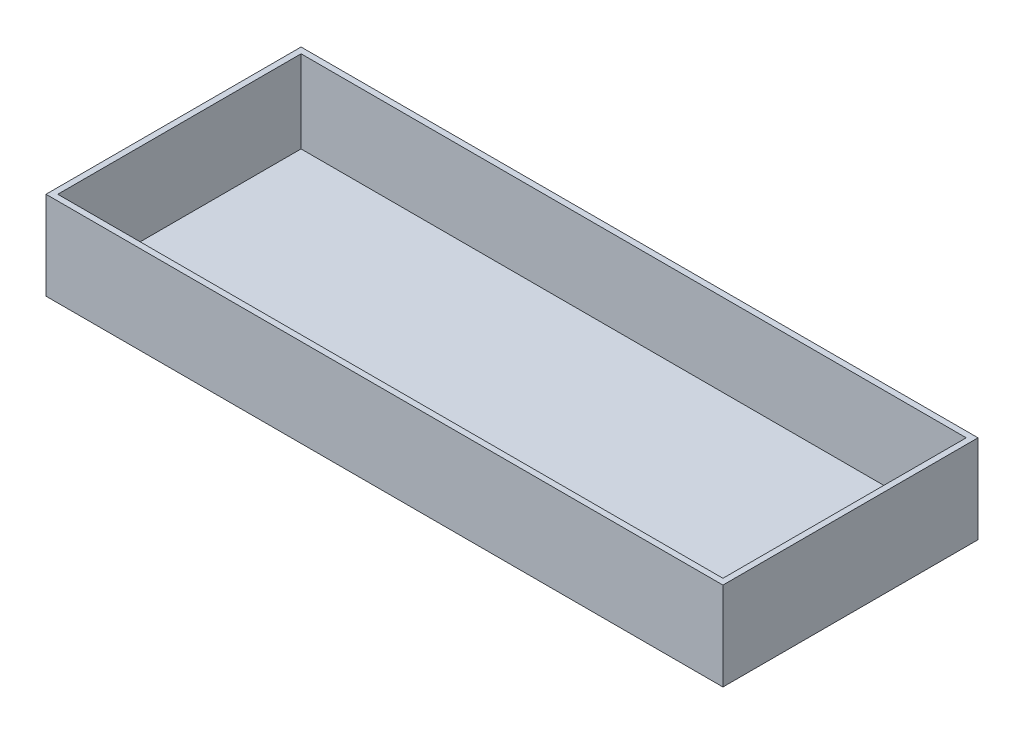
SolidWorks part; units mm, degrees
ref_plane "Front Plane" through (0, 0, 0) normal (0, 0, 1) x (1, 0, 0)
ref_plane "Top Plane" through (0, 0, 0) normal (0, 1, 0) x (1, 0, 0)
ref_plane "Right Plane" through (0, 0, 0) normal (1, 0, 0) x (0, 0, -1)
sketch "Sketch1" plane through (0, 0, 0) normal (0, 1, 0) x (1, 0, 0)
  line L1 (-345, 130) -> (345, 130)
  line L2 (-345, 130) -> (-345, -130)
  line L3 (-345, -130) -> (345, -130)
  line L4 (345, 130) -> (345, -130)
  line L5 (-345, 130) -> (345, -130) construction
  line L6 (-345, -130) -> (345, 130) construction
  point P0 (0, 0)
  dimension "D1" = 260
  dimension "D2" = 690
extrude "Boss-Extrude1" add sketch "Sketch1" along normal blind 90
shell "Shell1" thickness 6
